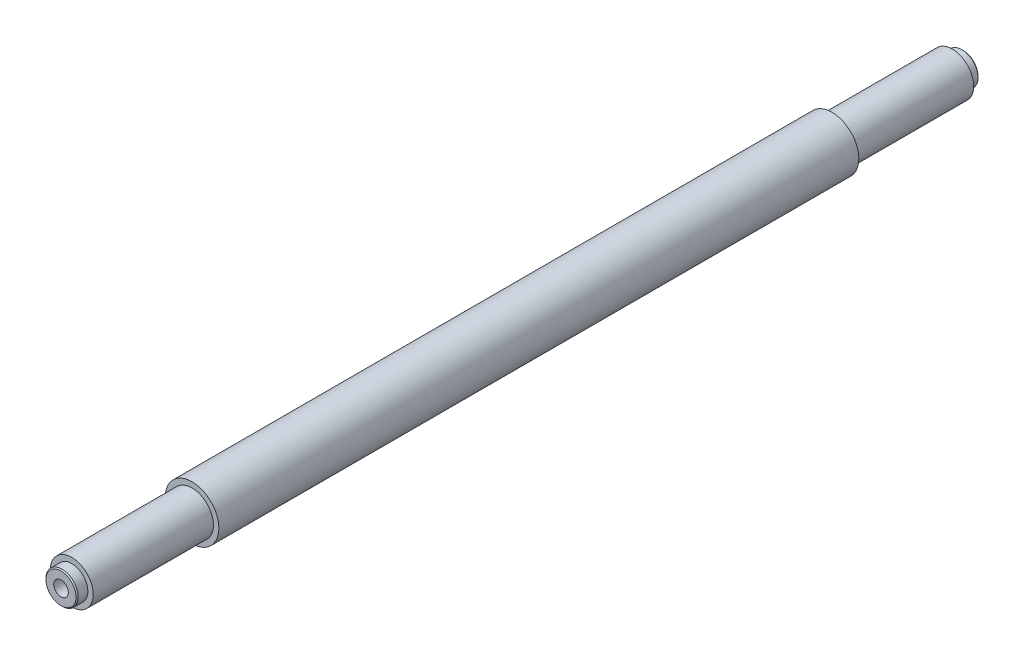
SolidWorks part; units mm, degrees
material "普通碳钢"
ref_plane "前视基准面" through (0, 0, 0) normal (0, 0, 1) x (1, 0, 0)
ref_plane "上视基准面" through (0, 0, 0) normal (0, 1, 0) x (1, 0, 0)
ref_plane "右视基准面" through (0, 0, 0) normal (1, 0, 0) x (0, 0, -1)
sketch "草图1" plane through (0, 0, 0) normal (0, 0, 1) x (1, 0, 0)
  circle A1 centre (0, 0) radius 12.5
  dimension "D2" = 25
extrude "凸台-拉伸1" add sketch "草图1" along normal blind 298
sketch "草图2" plane through (0, 0, 0) normal (0, 0, -1) x (-1, 0, 0)
  circle A0 centre (0, 0) radius 10
  dimension "D1" = 20
extrude "凸台-拉伸2" add sketch "草图2" along normal blind 56
sketch "草图3" plane through (0, 0, 298) normal (0, 0, 1) x (1, 0, 0)
  circle A0 centre (0, 0) radius 10
  dimension "D1" = 20
extrude "凸台-拉伸3" add sketch "草图3" along normal blind 56
sketch "草图4" plane through (0, 0, 354) normal (0, 0, 1) x (1, 0, 0)
  circle A0 centre (0, 0) radius 7.5
  dimension "D1" = 15
extrude "凸台-拉伸4" add sketch "草图4" along normal blind 5
sketch "草图5" plane through (0, 0, -56) normal (0, 0, -1) x (-1, 0, 0)
  circle A0 centre (0, 0) radius 7.5
  dimension "D1" = 15
extrude "凸台-拉伸5" add sketch "草图5" along normal blind 5
hole_wizard "M8 螺纹孔1" positions "草图7" profile "草图6" tap size "M8" standard "Iso"
sketch "草图7" plane through (0, 0, -61) normal (0, 0, -1) x (-1, 0, 0)
  point P0 (0, 0)
sketch "草图6" plane through (0, 0, -61) normal (1, 0, 0) x (0, 1, 0)
  line L0 (0, 0) -> (0, 21.7929)
  line L1 (0, 21.7929) -> (3.4, 19.75)
  line L2 (3.4, 19.75) -> (3.4, 0)
  line L5 (3.4, 0) -> (0, 0)
  line L10 (0, 21.7929) -> (-3.4, 19.75) construction
  line L11 (0, -6.35) -> (0, 107.95) construction
  dimension "螺纹孔钻头直径" = 6.8
  dimension "螺纹孔钻头深度" = 19.75
  dimension "导头角度" = 118
cosmetic thread "孔螺蚊线1" parameters "D1"=16, "D2"=8
hole_wizard "M8 螺纹孔2" positions "草图9" profile "草图8" tap size "M8" standard "Iso"
sketch "草图9" plane through (0, 0, 359) normal (0, 0, 1) x (1, 0, 0)
  point P0 (0, 0)
sketch "草图8" plane through (0, 0, 359) normal (1, 0, 0) x (0, -1, 0)
  line L0 (0, 0) -> (0, 21.7929)
  line L1 (0, 21.7929) -> (3.4, 19.75)
  line L2 (3.4, 19.75) -> (3.4, 0)
  line L5 (3.4, 0) -> (0, 0)
  line L10 (0, 21.7929) -> (-3.4, 19.75) construction
  line L11 (0, -6.35) -> (0, 107.95) construction
  dimension "螺纹孔钻头直径" = 6.8
  dimension "螺纹孔钻头深度" = 19.75
  dimension "导头角度" = 118
cosmetic thread "孔螺蚊线2" parameters "D1"=16, "D2"=8
chamfer "倒角2" distance 0.5 angle 45 1 edges at (7.5, 0, 359)
chamfer "倒角3" distance 0.5 angle 45 1 edges at (-7.5, 0, -61)
